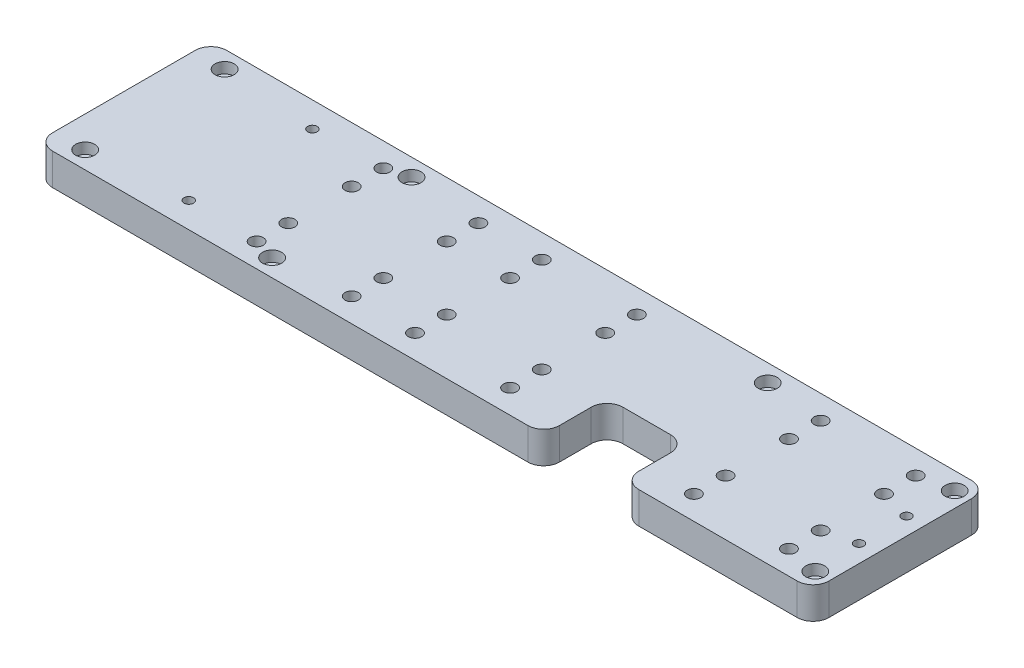
SolidWorks part; units mm, degrees
ref_plane "Front Plane" through (0, 0, 0) normal (0, 0, 1) x (1, 0, 0)
ref_plane "Top Plane" through (0, 0, 0) normal (0, 1, 0) x (1, 0, 0)
ref_plane "Right Plane" through (0, 0, 0) normal (1, 0, 0) x (0, 0, -1)
sketch "Sketch1" plane through (0, -16.8464, 0) normal (0, 1, 0) x (1, 0, 0)
  line L0 (67.5, -27.5) -> (117.5, -27.5)
  line L1 (-117.5, -27.5) -> (32.5, -27.5)
  line L2 (-122.5, -22.5) -> (-122.5, 22.5)
  line L3 (-117.5, 27.5) -> (117.5, 27.5)
  line L4 (122.5, -22.5) -> (122.5, 22.5)
  line L5 (-122.5, -27.5) -> (122.5, 27.5) construction
  line L6 (-122.5, 27.5) -> (122.5, -27.5) construction
  line L8 (37.5, -22.5) -> (37.5, -12.5)
  line L9 (42.5, -7.5) -> (57.5, -7.5)
  line L10 (62.5, -22.5) -> (62.5, -12.5)
  arc A0 (-117.5, -27.5) -> (-122.5, -22.5) centre (-117.5, -22.5) cw
  arc A1 (117.5, -27.5) -> (122.5, -22.5) centre (117.5, -22.5) ccw
  arc A2 (117.5, 27.5) -> (122.5, 22.5) centre (117.5, 22.5) cw
  arc A3 (-122.5, 22.5) -> (-117.5, 27.5) centre (-117.5, 22.5) cw
  arc A4 (32.5, -27.5) -> (37.5, -22.5) centre (32.5, -22.5) ccw
  arc A5 (67.5, -27.5) -> (62.5, -22.5) centre (67.5, -22.5) cw
  arc A6 (57.5, -7.5) -> (62.5, -12.5) centre (57.5, -12.5) cw
  arc A7 (37.5, -12.5) -> (42.5, -7.5) centre (42.5, -12.5) cw
  point P0 (0, 0)
  point P26 (62.5, -27.5)
  point P29 (62.5, -7.5)
  point P32 (37.5, -7.5)
  dimension "D6" = 5
  dimension "D7" = 5
  dimension "D1" = 245
  dimension "D2" = 55
  dimension "D3" = 160
  dimension "D4" = 25
  dimension "D5" = 20
extrude "Boss-Extrude1" add sketch "Sketch1" along normal blind 10
hole_wizard "CBORE for M3 Hexagon socket head cap screws1" positions "Sketch2" profile "Sketch3" counterbore size "M3" standard "GB"
sketch "Sketch2" plane through (0, -6.8464, 0) normal (0, 1, 0) x (1, 0, 0)
  line L2 (0, 0) -> (74.6894, 0) construction
  line L4 (114.2, 19.9378) -> (114.2, 23.9793) construction
  line L5 (117.5, 27.5) -> (-117.5, 27.5) construction
  line L6 (55.2, 19.9378) -> (55.2, 23.9793) construction
  line L7 (121.2, -19.9378) -> (121.2, -23.9793) construction
  line L8 (67.5, -27.5) -> (117.5, -27.5) construction
  line L9 (-117.5, -27.5) -> (32.5, -27.5) construction
  line L10 (-50.2, -19.9378) -> (-50.2, -23.9793) construction
  line L11 (0, 27.5) -> (0, -27.5) construction
  line L12 (0, -27.5) -> (0, -10.3797) construction
  line L13 (-50.2, 23.9793) -> (-50.2, 19.9378) construction
  line L14 (-109.2, 23.9793) -> (-109.2, 19.9378) construction
  line L15 (-109.2, -19.9378) -> (-109.2, -23.9793) construction
  point P0 (117.7, 22)
  point P14 (58.7, 22)
  point P23 (117.7, -22)
  point P30 (-53.7, -22)
  point P44 (-53.7, 22)
  point P46 (-112.7, 22)
  point P48 (-112.7, -22)
  dimension "D1" = 3.5
  dimension "D2" = 5.5
  dimension "D3" = 3.5
  dimension "D4" = 5.5
  dimension "D5" = 3.5
  dimension "D6" = 5.5
  dimension "D7" = 5.5
  dimension "D8" = 3.5
  dimension "D9" = 3.5
  dimension "D10" = 5.5
  dimension "D11" = 3.5
  dimension "D12" = 5.5
  dimension "D13" = 5.5
  dimension "D14" = 3.5
sketch "Sketch3" plane through (117.7, -6.8464, -22) normal (1, 0, 0) x (0, 0, 1)
  line L0 (0, 0) -> (0, 18.0215)
  line L1 (0, 18.0215) -> (1.7, 17)
  line L2 (1.7, 17) -> (1.7, 3.4)
  line L3 (1.7, 3.4) -> (3, 3.4)
  line L4 (3, 3.4) -> (3, 0)
  line L5 (3, 0) -> (0, 0)
  line L10 (0, 18.0215) -> (-1.7, 17) construction
  line L11 (0, -6.35) -> (0, 107.95) construction
  dimension "孔直径" = 3.4
  dimension "孔深度" = 17
  dimension "柱形沉头孔直径" = 6
  dimension "柱形沉头孔深度" = 3.4
  dimension "导头角度" = 118
hole_wizard "M5 Tapped Hole1" positions "Sketch4" profile "Sketch5" tap size "M5" standard "GB"
sketch "Sketch4" plane through (0, -6.8464, 0) normal (0, 1, 0) x (1, 0, 0)
  line L0 (-70.6, 20) -> (-21, 20) construction
  line L2 (-70.6, -20) -> (117, -20) construction
  line L4 (67.4, 20) -> (117, 20) construction
  line L5 (0, 0) -> (-122.5, 0) construction
  line L6 (-122.5, 22.5) -> (-122.5, -22.5) construction
  arc A0 (-68.3, 22.3) -> (-68.3, 17.7) centre (-68.3, 20) ccw construction
  arc A1 (-23.3, 17.7) -> (-23.3, 22.3) centre (-23.3, 20) ccw construction
  arc A2 (-68.3, -17.7) -> (-68.3, -22.3) centre (-68.3, -20) ccw construction
  arc A3 (114.7, -22.3) -> (114.7, -17.7) centre (114.7, -20) ccw construction
  arc A4 (69.7, 22.3) -> (69.7, 17.7) centre (69.7, 20) ccw construction
  arc A5 (114.7, 17.7) -> (114.7, 22.3) centre (114.7, 20) ccw construction
  point P32 (-60.6, 20)
  point P34 (-30.6, 20)
  point P36 (-60.6, -20)
  point P38 (-30.6, -20)
  point P40 (77.4, 20)
  point P42 (107.4, 20)
  point P44 (77.4, -20)
  point P46 (107.4032, -20)
  point P63 (-30.6, 10)
  point P65 (-60.6, 10)
  point P84 (77.4, 10)
  point P86 (107.4, 10)
  point P92 (107.4, -10)
  point P93 (77.4, -10)
  point P94 (-30.6, -10)
  point P95 (-60.6, -10)
  dimension "D1" = 30
  dimension "D2" = 10
  dimension "D3" = 10
  dimension "D4" = 30
  dimension "D5" = 10
  dimension "D6" = 30
  dimension "D7" = 30.0032
  dimension "D8" = 10
sketch "Sketch5" plane through (-60.6, -6.8464, 10) normal (1, 0, 0) x (0, 0, 1)
  line L0 (0, 0) -> (0, 15.2618)
  line L1 (0, 15.2618) -> (2.1, 14)
  line L2 (2.1, 14) -> (2.1, 0)
  line L5 (2.1, 0) -> (0, 0)
  line L10 (0, 15.2618) -> (-2.1, 14) construction
  line L11 (0, -6.35) -> (0, 107.95) construction
  dimension "螺纹孔钻头直径" = 4.2
  dimension "螺纹孔钻头深度" = 14
  dimension "导头角度" = 118
cosmetic thread "Cosmetic Thread1" parameters "D1"=10, "D2"=5
cosmetic thread "Cosmetic Thread2" parameters "D1"=10, "D2"=5
cosmetic thread "Cosmetic Thread3" parameters "D1"=10, "D2"=5
cosmetic thread "Cosmetic Thread4" parameters "D1"=10, "D2"=5
cosmetic thread "Cosmetic Thread5" parameters "D1"=10, "D2"=5
cosmetic thread "Cosmetic Thread6" parameters "D1"=10, "D2"=5
cosmetic thread "Cosmetic Thread7" parameters "D1"=10, "D2"=5
cosmetic thread "Cosmetic Thread8" parameters "D1"=10, "D2"=5
cosmetic thread "Cosmetic Thread9" parameters "D1"=10, "D2"=5
cosmetic thread "Cosmetic Thread10" parameters "D1"=10, "D2"=5
cosmetic thread "Cosmetic Thread11" parameters "D1"=10, "D2"=5
cosmetic thread "Cosmetic Thread12" parameters "D1"=10, "D2"=5
cosmetic thread "Cosmetic Thread13" parameters "D1"=10, "D2"=5
cosmetic thread "Cosmetic Thread14" parameters "D1"=10, "D2"=5
cosmetic thread "Cosmetic Thread15" parameters "D1"=10, "D2"=5
cosmetic thread "Cosmetic Thread16" parameters "D1"=10, "D2"=5
sketch "Sketch6" plane through (0, -16.8464, 0) normal (0, -1, 0) x (1, 0, 0)
  circle A0 centre (-82.5, 19.5) radius 1.5
  circle A1 centre (-82.5, -19.5) radius 1.5
  circle A2 centre (117, 7.5) radius 1.5
  circle A3 centre (117, -7.5) radius 1.5
  dimension "D1" = 3
  dimension "D2" = 3
  dimension "D3" = 3
  dimension "D4" = 3
extrude "Cut-Extrude1" cut sketch "Sketch6" against normal through all
pattern_linear "LPattern1" count 2 spacing 50 along (1, 0, 0) of "M5 Tapped Hole1"
cosmetic thread "Cosmetic Thread17" parameters "D1"=10, "D2"=5
cosmetic thread "Cosmetic Thread18" parameters "D1"=10, "D2"=5
cosmetic thread "Cosmetic Thread19" parameters "D1"=10, "D2"=5
cosmetic thread "Cosmetic Thread20" parameters "D1"=10, "D2"=5
cosmetic thread "Cosmetic Thread21" parameters "D1"=10, "D2"=5
cosmetic thread "Cosmetic Thread22" parameters "D1"=10, "D2"=5
cosmetic thread "Cosmetic Thread23" parameters "D1"=10, "D2"=5
cosmetic thread "Cosmetic Thread24" parameters "D1"=10, "D2"=5
equation "\"1\"= \"代号代号\""
equation "\"2\"= \"名称代号\""
